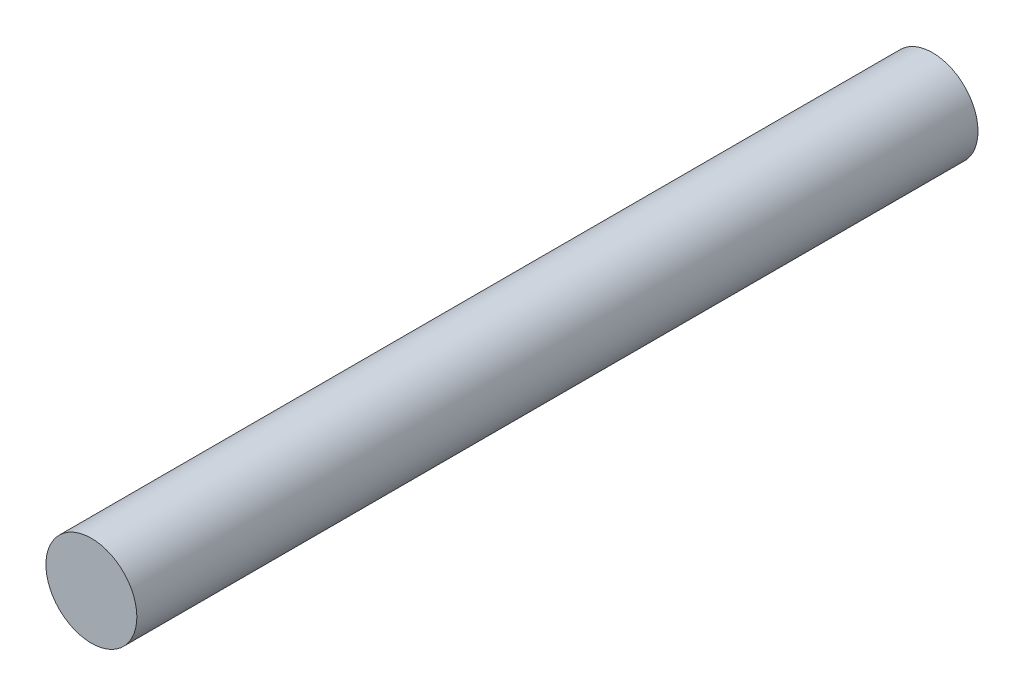
from build123d import *

# Parameters (mm, degrees)
SKETCH_1_R      = 2
EXTRUDE_1_DEPTH = 37


with BuildPart() as part:
    # 草图1 → 凸台-拉伸1 (new body)
    with BuildSketch(Plane.XY):
        Circle(SKETCH_1_R)
    extrude(amount=EXTRUDE_1_DEPTH)


solid = part.part
